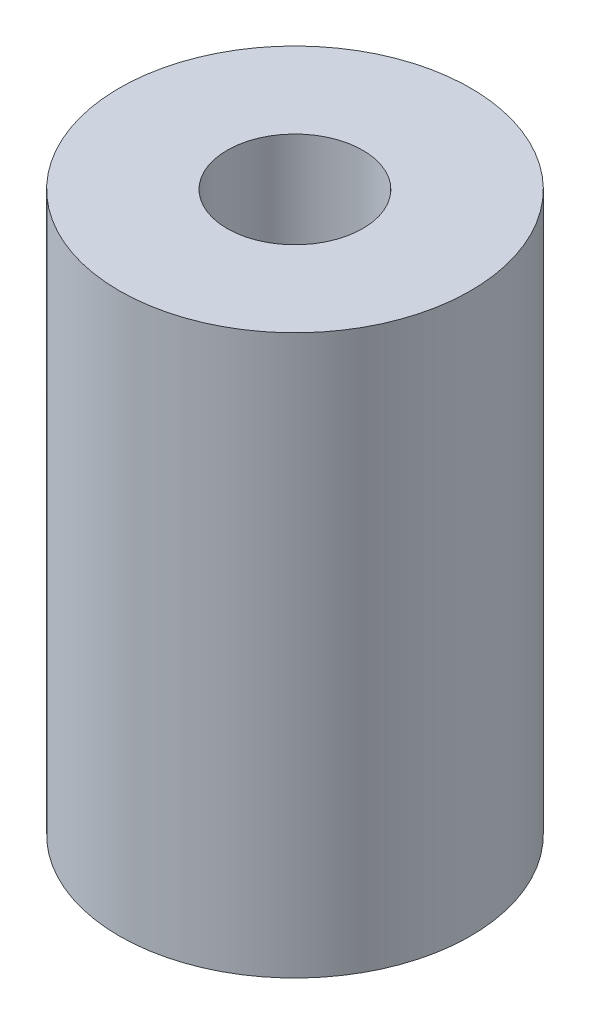
from build123d import *

# Parameters (mm, degrees)
SKETCH1_R           = 11
BOSS_EXTRUDE1_DEPTH = 35
M10_TAPPED_HOLE1_D  = 8.5


with BuildPart() as part:
    # Sketch1 → Boss-Extrude1 (new body)
    with BuildSketch(Plane(origin=(0, 0, 0), x_dir=(1, 0, 0), z_dir=(0, 1, 0))):
        with Locations(Location((0, 0, 0), (0, 0, 270))):
            Circle(SKETCH1_R)
    extrude(amount=BOSS_EXTRUDE1_DEPTH)

    # M10 Tapped Hole1 (through all)
    with Locations(Plane(origin=(0, 35, 0), x_dir=(1, 0, 0), z_dir=(0, 1, 0))):
        with Locations((0, 0)):
            Hole(M10_TAPPED_HOLE1_D / 2)


solid = part.part
